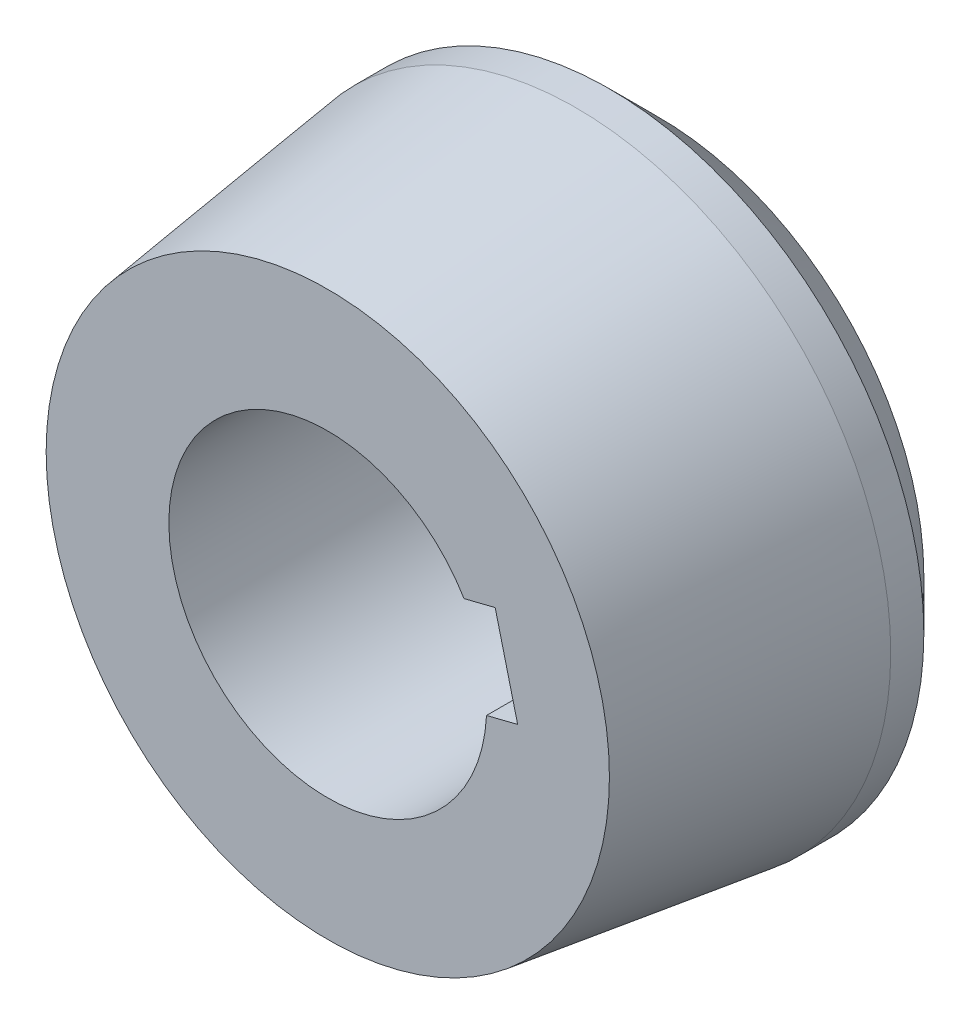
from build123d import *

# Parameters (mm, degrees)
CUT_EXTRUDE1_DEPTH = 637.880050586
SKETCH3_W          = 24
SKETCH3_H          = 50


with BuildPart() as part:
    # Sketch1 → Revolve1 (revolve)
    with BuildSketch(Plane(origin=(0, 234.743963655, 0), x_dir=(1, 0, 0), z_dir=(0, 1, 0))):
        Polygon((561.230642584, 824.998443067), (521.230642584, 824.998443067), (521.230642584, 774.998443067), (563.755642584, 774.998443067), (568.730642584, 812.498443067), (568.730642584, 817.498443067), align=None)
    revolve(axis=Axis((521.230642584, 234.743963655, -824.998443067), (0, 0, 1)))

    # Sketch2 → Cut-Extrude1 (cut, through all)
    with BuildSketch(Plane.XY.offset(-774.998443067)):
        with BuildLine():
            Line((549.898349026, 234.692901362), (546.50406086, 248.275198952))
            Line((546.50406086, 248.275198952), (541.805052122, 247.10089176))
            ThreePointArc((541.805052122, 247.10089176), (544.514581311, 240.562743369), (545.199340288, 233.518594169))
            Line((545.199340288, 233.518594169), (549.898349026, 234.692901362))
        make_face()
    extrude(amount=-CUT_EXTRUDE1_DEPTH, mode=Mode.SUBTRACT)

    # Sketch3 → Cut-Revolve1 (revolve, cut)
    with BuildSketch(Plane.XZ.offset(-234.743963655)):
        with Locations((533.230642584, -799.998443067)):
            Rectangle(SKETCH3_W, SKETCH3_H)
    revolve(axis=Axis((521.230642584, 234.743963655, -774.998443067), (0, 0, -1)), mode=Mode.SUBTRACT)


solid = part.part
